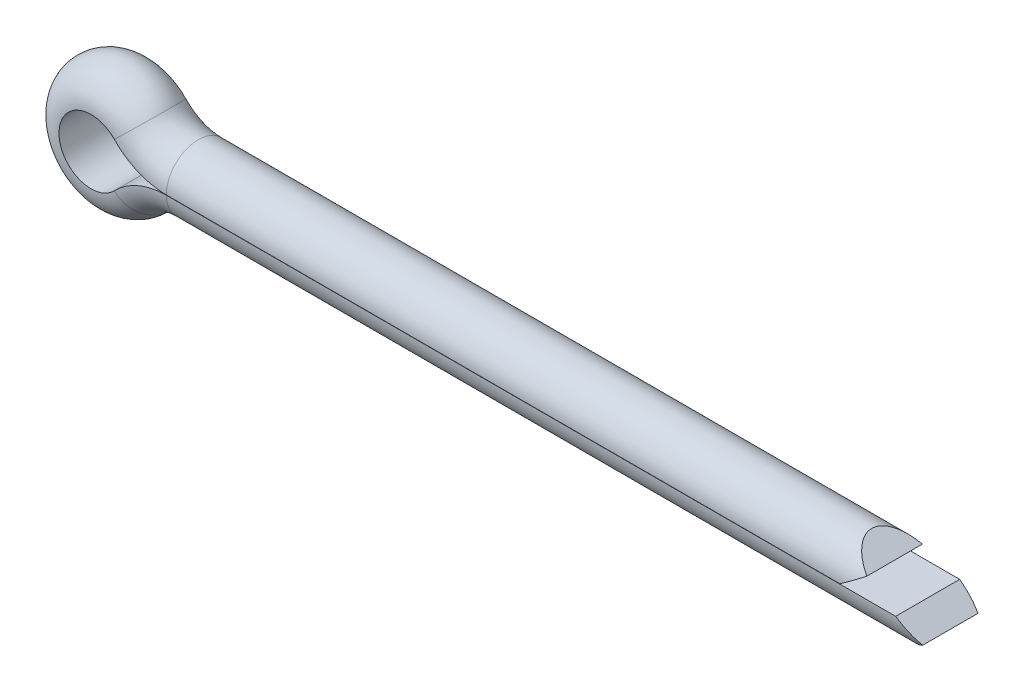
SolidWorks part; units mm, degrees
ref_plane "前视基准面" through (0, 0, 0) normal (0, 0, 1) x (1, 0, 0)
ref_plane "上视基准面" through (0, 0, 0) normal (0, 1, 0) x (1, 0, 0)
ref_plane "右视基准面" through (0, 0, 0) normal (1, 0, 0) x (0, 0, -1)
sketch "尺寸草图" plane through (0, 0, 0) normal (0, 0, 1) x (1, 0, 0)
  line L0 (55.4, 2.3) -> (5.4, 2.3)
  line L1 (5.4, -2.3) -> (59.4, -2.3)
  line L2 (5.4, 0) -> (27.3859, 0) construction
  line L3 (5.4, 0) -> (5.4, -0.0723) construction
  line L4 (-4.6, 0) -> (-4.6, 18.8979) construction
  arc A0 (5.4, 2.3) -> (3.3168, 3.1873) centre (5.4, 5.1891) cw
  arc A1 (3.3168, 3.1873) -> (3.3168, -3.1873) centre (0, 0) ccw
  arc A2 (3.3168, -3.1873) -> (5.4, -2.3) centre (5.4, -5.1891) cw
  dimension "c" = 9.2
  dimension "d1" = 4.6
  dimension "b" = 10
  dimension "l" = 50
  dimension "a" = 4
ref_plane "基准面1" through (55.4, 2.3, 0) normal (-1, 0, 0) x (0, 0, 1)
sketch "草图2" plane through (55.4, 2.3, 0) normal (-1, 0, 0) x (0, 0, 1)
  line L0 (0, -6.9) -> (0, 2.3) construction
  line L1 (-2.3, -2.29) -> (2.3, -2.29)
  arc A0 (2.3, -2.29) -> (-2.3, -2.29) centre (0, -2.3) ccw
  dimension "d" = 4.6
  dimension "D1" = 0.01
sweep "扫描2" add profiles "草图2" path "尺寸草图"
sketch "草图3" plane through (0, 0, 0) normal (0, 0, 1) x (1, 0, 0)
  line L0 (5.4, 0) -> (5.4, 16.2682) construction
  line L1 (5.4, 0) -> (37.4999, 0) construction
  line L2 (59.4, -2.3) -> (59.4, -0.01) construction
  line L3 (55.4, 1.145) -> (53.7611, 2.3)
  line L4 (55.4, 2.3) -> (5.4, 2.3) construction
  line L5 (5.4, -2.3) -> (59.4, -2.3) construction
  line L6 (55.4, 1.145) -> (53.7541, 0)
  line L7 (59.4, -1.155) -> (57.7611, 0)
  line L9 (59.4, -1.155) -> (57.7541, -2.3)
  line L10 (57.7611, 0) -> (53.7541, 0)
  line L11 (53.7611, 2.3) -> (59.41, 2.3)
  line L12 (59.41, 2.3) -> (59.41, -2.3)
  line L13 (59.41, -2.3) -> (57.7541, -2.3)
  line L14 (55.4, 2.3) -> (55.4, 0.01) construction
  dimension "D1" = 0.01
  dimension "D3" = 70
  dimension "D4" = 70
extrude "切除-拉伸1" cut sketch "草图3" against normal through all and the other way through all
